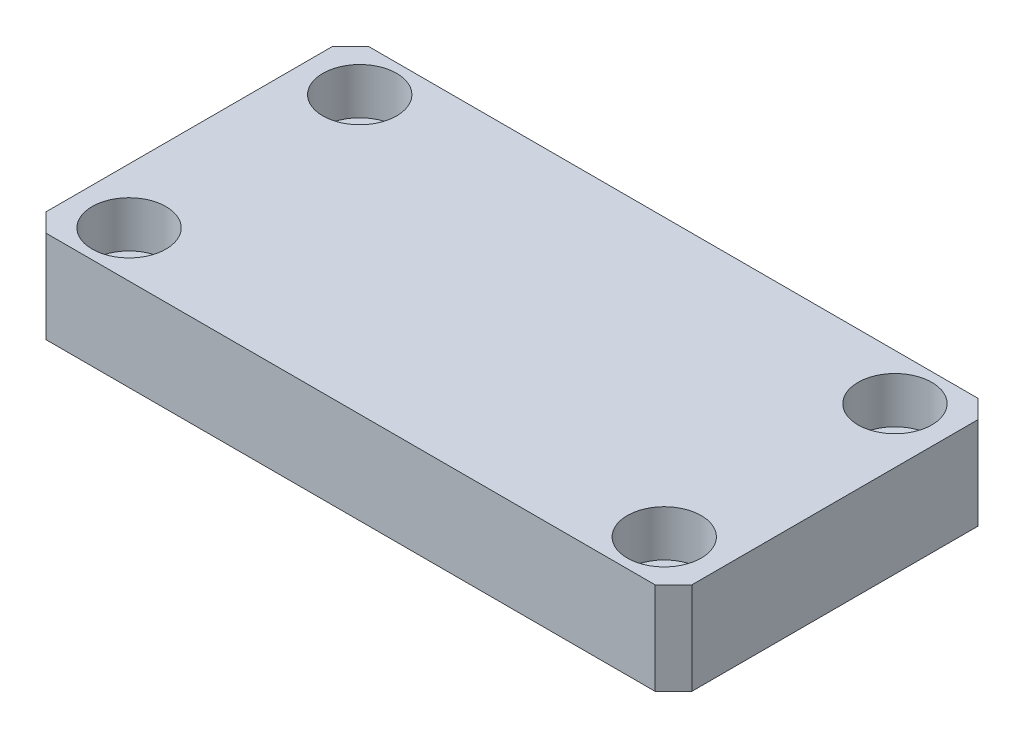
from build123d import *

# Parameters (mm, degrees)
SKETCH_1_W                   = 70
SKETCH_1_H                   = 35
EXTRUDE_1_DEPTH              = 5
CHAMFER_1_SIZE               = 2
HOLE_WIZARD_M4_1_D           = 4.5
HOLE_WIZARD_M4_1_CBORE_D     = 8
HOLE_WIZARD_M4_1_CBORE_DEPTH = 5


with BuildPart() as part:
    # 草图1 → 凸台-拉伸1 (new, symmetric)
    with BuildSketch(Plane(origin=(0, 0, 0), x_dir=(1, 0, 0), z_dir=(0, 1, 0))):
        Rectangle(SKETCH_1_W, SKETCH_1_H)
    extrude(amount=EXTRUDE_1_DEPTH, both=True)

    # 倒角1
    chamfer_1_edges = [part.edges().sort_by_distance(p)[0] for p in [
        (35, 0, 17.5),
        (-35, 0, 17.5),
        (-35, 0, -17.5),
        (35, 0, -17.5),
    ]]
    chamfer(chamfer_1_edges, length=CHAMFER_1_SIZE)

    # M4 六角圆柱头螺钉的柱形沉头孔1 (through all)
    with Locations(Plane(origin=(0, 5, 0), x_dir=(1, 0, 0), z_dir=(0, 1, 0))):
        with Locations((-29, 12.5), (-29, -12.5), (29, 12.5), (29, -12.5)):
            CounterBoreHole(HOLE_WIZARD_M4_1_D / 2, HOLE_WIZARD_M4_1_CBORE_D / 2, HOLE_WIZARD_M4_1_CBORE_DEPTH)


solid = part.part
